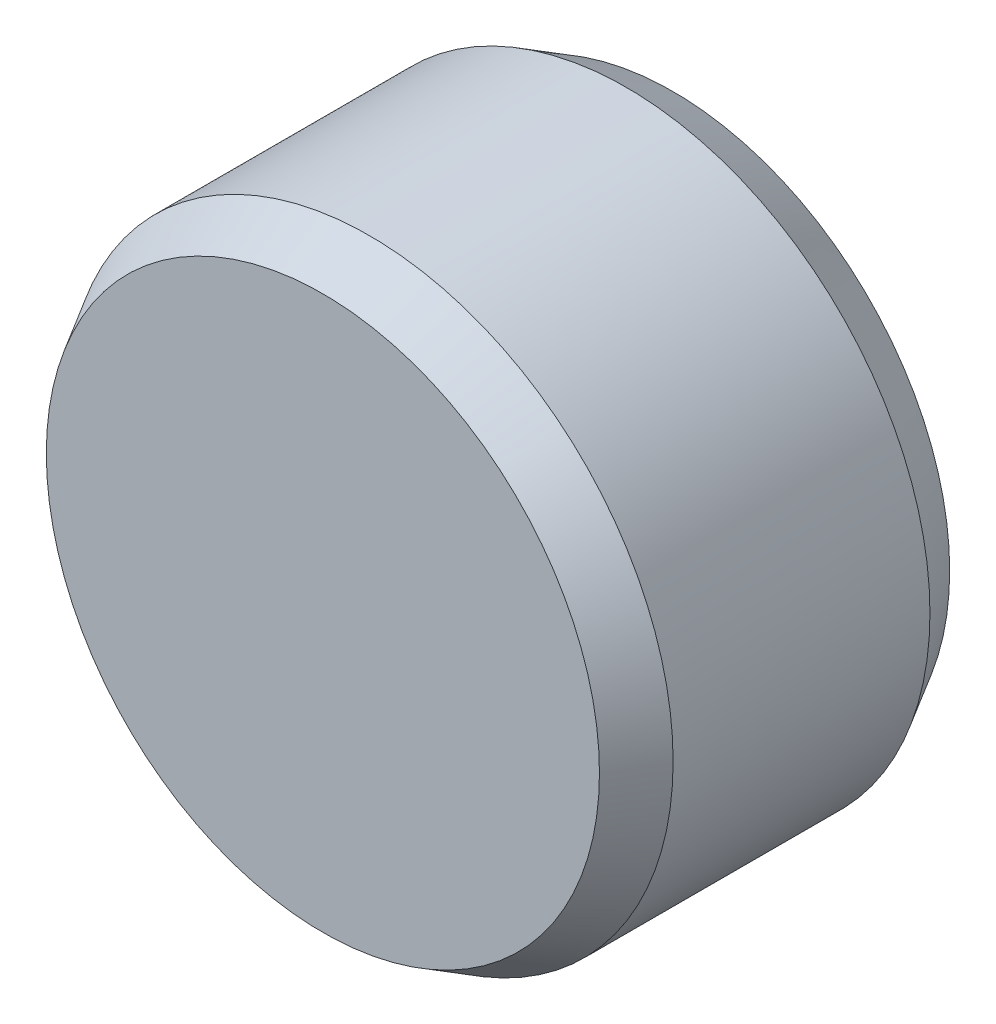
SolidWorks part; units mm, degrees
material "Q345 "
ref_plane "前视基准面" through (0, 0, 0) normal (0, 0, 1) x (1, 0, 0)
ref_plane "上视基准面" through (0, 0, 0) normal (0, 1, 0) x (1, 0, 0)
ref_plane "右视基准面" through (0, 0, 0) normal (1, 0, 0) x (0, 0, -1)
sketch "草图1" plane through (0, 0, 0) normal (0, 0, 1) x (1, 0, 0)
  circle A0 centre (0, 0) radius 65
  dimension "D1" = 130
extrude "凸台-拉伸1" add sketch "草图1" along normal blind 75
chamfer "倒角1" distance 10 angle 30 2 edges at (65, 0, 0) (65, 0, 75)
